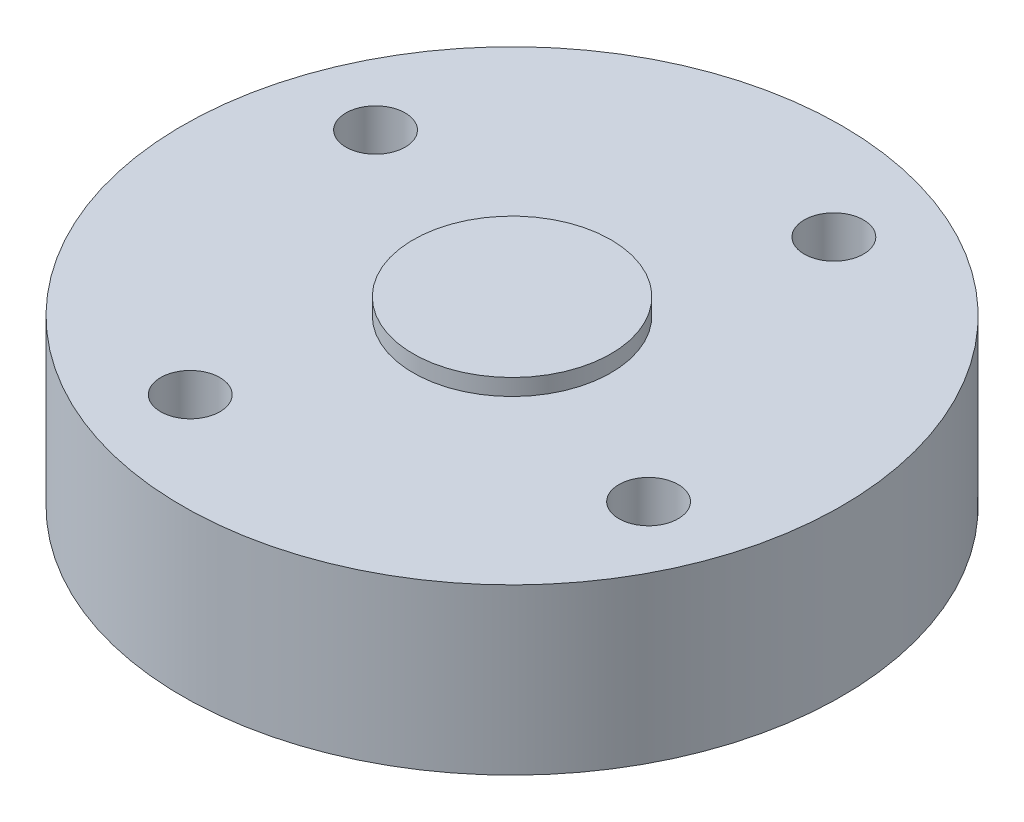
from build123d import *

# Parameters (mm, degrees)
F_18_0_18_DIAMETER_HOLE1_D     = 18
F_18_0_18_DIAMETER_HOLE1_DEPTH = 90


with BuildPart() as part:
    # Sketch1 → Revolve1 (revolve)
    with BuildSketch(Plane.XY, mode=Mode.PRIVATE) as revolve1_sk:
        Polygon((30, -31.6), (100, -31.6), (100, -81.6), (25, -81.6), (25, -121.6), (0, -121.6), (0, -26.6), (30, -26.6), align=None)
    revolve(revolve1_sk.sketch.rotate(Axis((0, 0, 0), (0, 1, 0)), 90), axis=Axis((0, 0, 0), (0, 1, 0)))

    # Ø18.0 (18) Diameter Hole1
    with Locations(Plane(origin=(0, -31.6, 0), x_dir=(1, 0, 0), z_dir=(0, 1, 0))):
        with Locations((-69.533343678, 28.108968621), (-28.108968621, -69.533343678), (69.533343678, -28.108968621), (28.108968621, 69.533343678)):
            Hole(F_18_0_18_DIAMETER_HOLE1_D / 2, depth=F_18_0_18_DIAMETER_HOLE1_DEPTH)


solid = part.part
